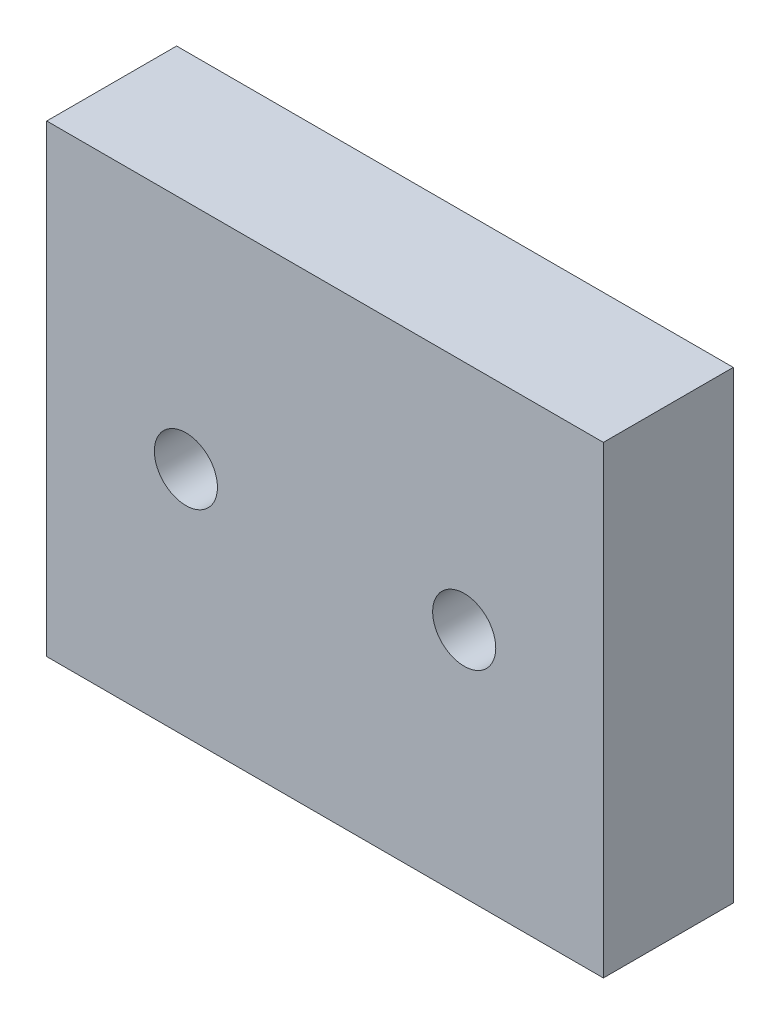
SolidWorks part; units mm, degrees
material "Q235"
ref_plane "Front" through (0, 0, 0) normal (0, 0, 1) x (1, 0, 0)
ref_plane "Top" through (0, 0, 0) normal (0, 1, 0) x (1, 0, 0)
ref_plane "Right" through (0, 0, 0) normal (1, 0, 0) x (0, 0, -1)
sketch "Sketch1" plane through (0, 0, 0) normal (0, 0, 1) x (1, 0, 0)
  line L1 (-30, 25) -> (30, 25)
  line L2 (-30, 25) -> (-30, -25)
  line L3 (-30, -25) -> (30, -25)
  line L4 (30, 25) -> (30, -25)
  line L5 (-30, 25) -> (30, -25) construction
  line L6 (-30, -25) -> (30, 25) construction
  point P0 (0, 0)
  dimension "D1" = 60
  dimension "D2" = 50
extrude "Boss-Extrude1" add sketch "Sketch1" along normal blind 14
hole_wizard "M8 Tapped Hole1" positions "Sketch2" profile "Sketch3" tap size "M8" standard "GB"
sketch "Sketch2" plane through (0, 0, 14) normal (0, 0, 1) x (1, 0, 0)
  line L0 (0, -25) -> (0, -15.2396) construction
  line L1 (-30, -25) -> (30, -25) construction
  point P0 (-15, 0)
  point P2 (15, 0)
  dimension "D1" = 30
  dimension "D2" = 25
sketch "Sketch3" plane through (-15, 0, 14) normal (1, 0, 0) x (0, -1, 0)
  line L0 (0, 0) -> (0, 21.7929)
  line L1 (0, 21.7929) -> (3.4, 19.75)
  line L2 (3.4, 19.75) -> (3.4, 0)
  line L5 (3.4, 0) -> (0, 0)
  line L10 (0, 21.7929) -> (-3.4, 19.75) construction
  line L11 (0, -6.35) -> (0, 107.95) construction
  dimension "螺纹孔钻头直径" = 6.8
  dimension "螺纹孔钻头深度" = 19.75
  dimension "导头角度" = 118
cosmetic thread "Hole Cosmetic Thread1" parameters "D1"=14, "D2"=8
cosmetic thread "Hole Cosmetic Thread2" parameters "D1"=14, "D2"=8
